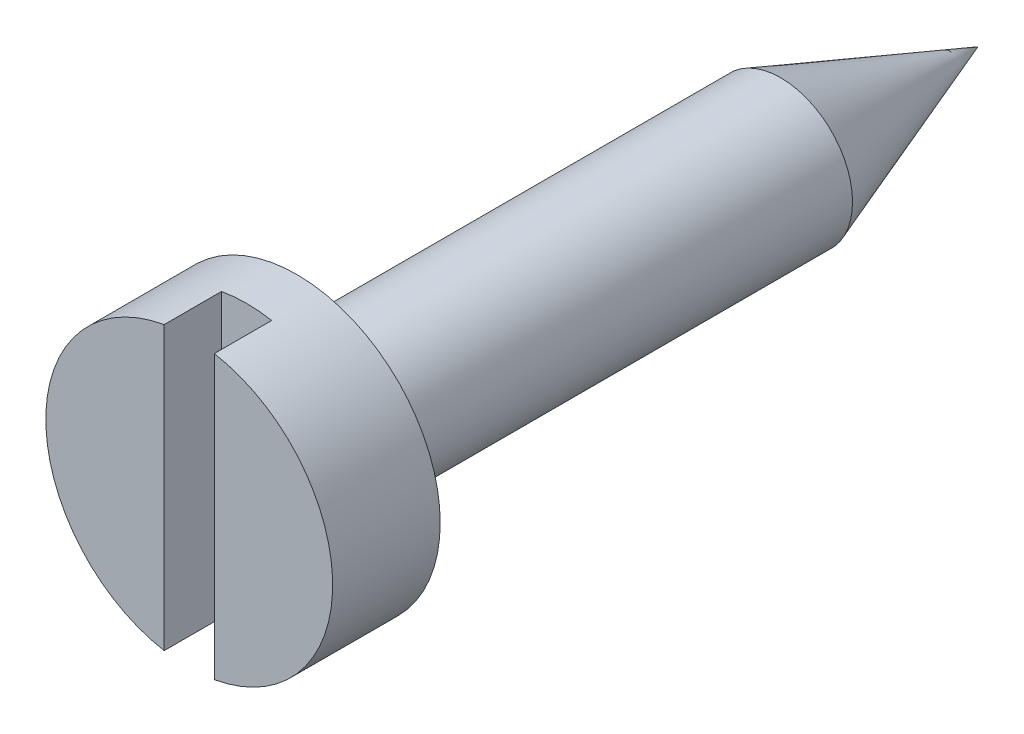
SolidWorks part; units mm, degrees
ref_plane "Front Plane" through (0, 0, 0) normal (0, 0, 1) x (1, 0, 0)
ref_plane "Top Plane" through (0, 0, 0) normal (0, 1, 0) x (1, 0, 0)
ref_plane "Right Plane" through (0, 0, 0) normal (1, 0, 0) x (0, 0, -1)
other "Configuration Table"
sketch "Sketch1" plane through (0, 0, 0) normal (0, 0, 1) x (1, 0, 0)
  circle A0 centre (0, 0) radius 4
  dimension "D1" = 8
extrude "Boss-Extrude1" add sketch "Sketch1" along normal blind 3
sketch "Sketch2" plane through (0, 0, 3) normal (0, 0, 1) x (1, 0, 0)
  line L1 (0.7, 4.8277) -> (-0.7, 4.8277)
  line L2 (0.7, 4.8277) -> (0.7, -4.8277)
  line L3 (0.7, -4.8277) -> (-0.7, -4.8277)
  line L4 (-0.7, 4.8277) -> (-0.7, -4.8277)
  line L5 (0.7, 4.8277) -> (-0.7, -4.8277) construction
  line L6 (0.7, -4.8277) -> (-0.7, 4.8277) construction
  point P0 (0, 0)
  dimension "D1" = 1.4
extrude "Cut-Extrude1" cut sketch "Sketch2" against normal blind 1.6
sketch "Sketch3" plane through (0, 0, 0) normal (0, 0, -1) x (-1, 0, 0)
  circle A0 centre (0, 0) radius 2
  dimension "D1" = 4
extrude "Boss-Extrude2" add sketch "Sketch3" along normal blind 19
cosmetic thread "Cosmetic Thread1" parameters "D2"=3
sketch "Sketch4" plane through (0, 0, 0) normal (0, 1, 0) x (1, 0, 0)
  line L0 (0, 19) -> (0, -49981) construction
  line L4 (2, 0) -> (2, 19) construction
  line L8 (2, 19) -> (-2, 19) construction
  line L10 (2, 13.5) -> (2, 19)
  line L13 (2, 19) -> (0, 26.1827)
  line L15 (2, 13.5) -> (0, 19)
  line L16 (0, 19) -> (0, 26.1827)
  point P5 (0, 19)
  dimension "D1" = 5.5
revolve "Cut-Revolve5" cut sketch "Sketch4" angle 360 about L0
